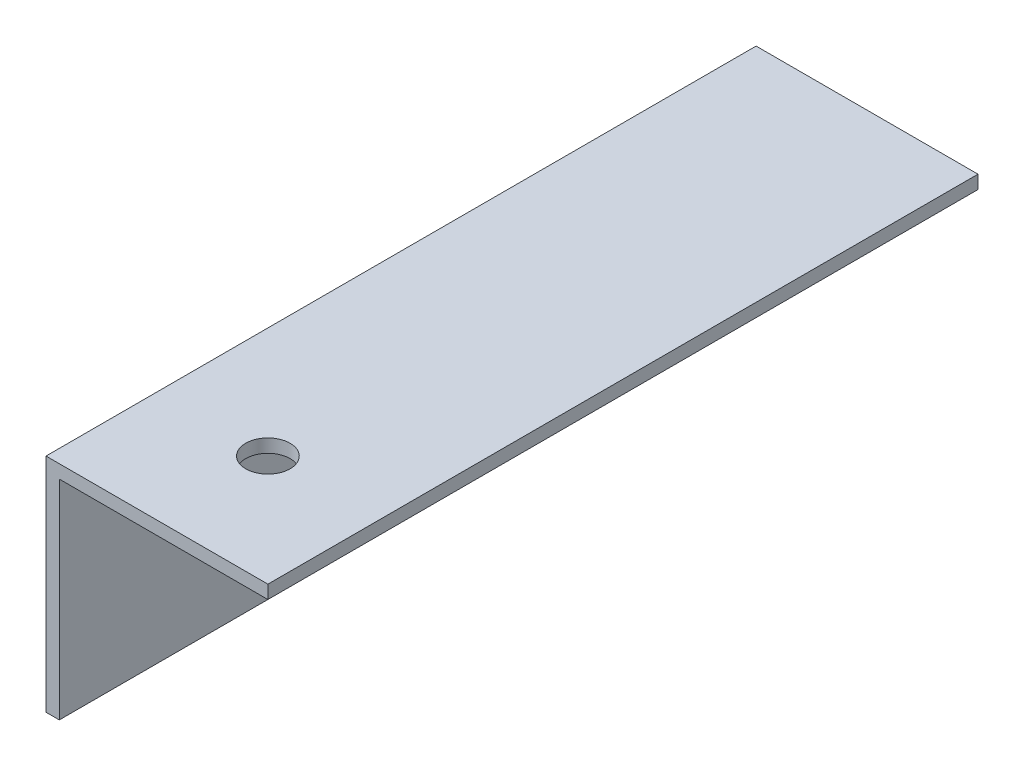
SolidWorks part; units mm, degrees
ref_plane "前视基准面" through (0, 0, 0) normal (0, 0, 1) x (1, 0, 0)
ref_plane "上视基准面" through (0, 0, 0) normal (0, 1, 0) x (1, 0, 0)
ref_plane "右视基准面" through (0, 0, 0) normal (1, 0, 0) x (0, 0, -1)
sketch "草图1" plane through (0, 0, 0) normal (0, 0, 1) x (1, 0, 0)
  line L0 (0, 0) -> (-50, 0)
  line L1 (-50, 0) -> (-50, -50)
  line L2 (0, -3) -> (-47, -3)
  line L3 (-47, -3) -> (-47, -50)
  line L4 (0, -3) -> (0, 0)
  line L5 (-50, -50) -> (-47, -50)
  dimension "D1" = 3
extrude "凸台-拉伸1" add sketch "草图1" along normal blind 160
sketch "草图2" plane through (0, 0, 0) normal (0, 1, 0) x (1, 0, 0)
  line L0 (0, -160) -> (0, -110)
  line L1 (0, -160) -> (0, 0) construction
  line L2 (0, -110) -> (-50, -110)
  line L3 (-50, -160) -> (-50, 0) construction
  line L4 (-50, -110) -> (0, -160)
  circle A0 centre (-25, -135) radius 5
extrude "切除-拉伸1" cut sketch "草图2" against normal blind 10 contours L4 A0 | L4 A0
